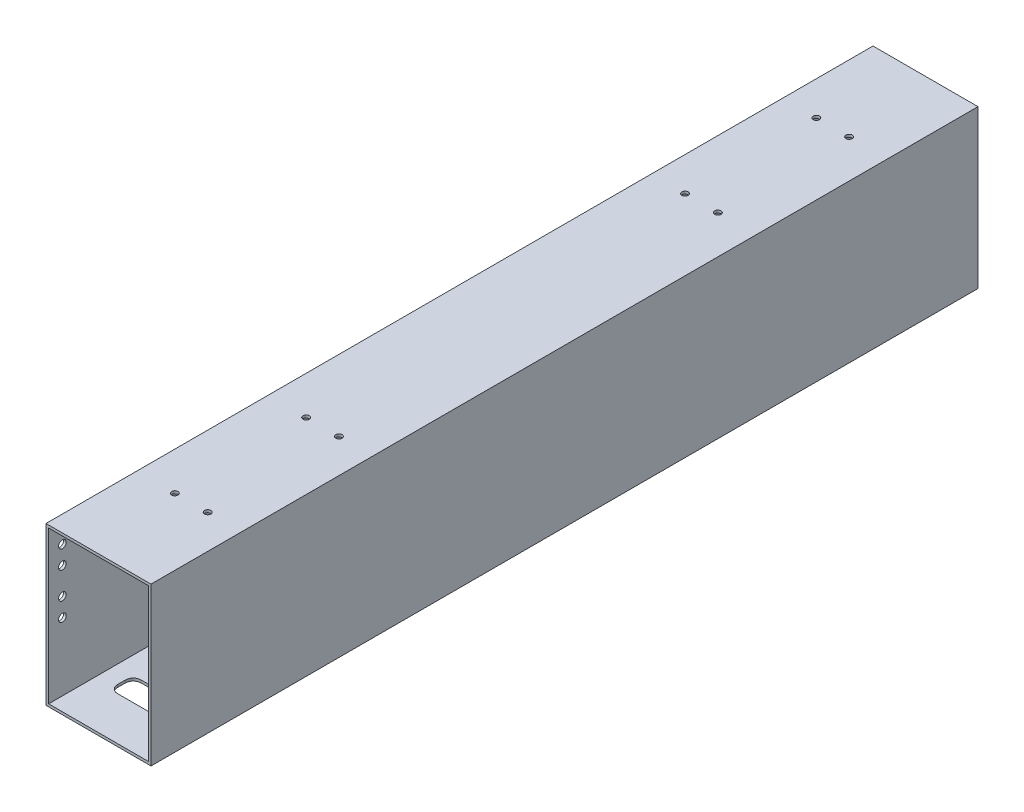
from build123d import *

# Parameters (mm, degrees)
SKETCH_1_W             = 80
SKETCH_1_H             = 120
SKETCH_1_W_2           = 76
SKETCH_1_H_2           = 116
EXTRUDE_1_DEPTH        = 315
CUT_EXTRUDE_2_REACH    = 332.492
SKETCH_4_R             = 25
HOLE_WIZARD_M5_1_D     = 5.8
HOLE_WIZARD_M5_1_DEPTH = 2
HOLE_WIZARD_M4_1_D     = 4.8
HOLE_WIZARD_M4_1_DEPTH = 2
CUT_EXTRUDE_3_REACH    = 341.448
SKETCH_15_W            = 50
SKETCH_15_H            = 18
SKETCH_15_W_2          = 60
SKETCH_15_H_2          = 75
FILLET_1_R             = 6


with BuildPart() as part:
    # 草图1 → 拉伸-薄壁1 (new, symmetric)
    with BuildSketch(Plane.XY):
        Rectangle(SKETCH_1_W, SKETCH_1_H)
        Rectangle(SKETCH_1_W_2, SKETCH_1_H_2, mode=Mode.SUBTRACT)
    extrude(amount=EXTRUDE_1_DEPTH, both=True)

    # 草图4 → 切除-拉伸2 (cut, up to next)
    with BuildSketch(Plane.ZY.offset(40), mode=Mode.PRIVATE) as cut_extrude_2_sk1:
        with Locations((0, -20)):
            Circle(SKETCH_4_R)
    cut_extrude_2_tool1 = extrude(cut_extrude_2_sk1.sketch, amount=-CUT_EXTRUDE_2_REACH, mode=Mode.PRIVATE) & part.part
    add(cut_extrude_2_tool1.solids().sort_by_distance((-40, -20, 0))[0], mode=Mode.SUBTRACT)

    # M5 间隙孔1
    with Locations(Plane.ZY.offset(40)):
        with Locations((304.5, 42), (304.5, 28), (304.5, 7.61), (304.5, -6.39), (-304.5, -6.39), (-304.5, 7.61), (-304.5, 28), (-304.5, 42)):
            Hole(HOLE_WIZARD_M5_1_D / 2, depth=HOLE_WIZARD_M5_1_DEPTH)

    # M4 间隙孔1
    with Locations(Plane(origin=(0, 60, 0), x_dir=(1, 0, 0), z_dir=(0, 1, 0))):
        with Locations((-14.175, 246), (10.825, 246), (-14.175, 146), (10.825, 146), (-10.825, -146), (14.175, -146), (-10.825, -246), (14.175, -246)):
            Hole(HOLE_WIZARD_M4_1_D / 2, depth=HOLE_WIZARD_M4_1_DEPTH)

    # 草图15 → 切除-拉伸3 (cut, up to next)
    with BuildSketch(Plane.XZ.offset(60), mode=Mode.PRIVATE) as cut_extrude_3_sk1:
        with Locations((0.475, -273)):
            Rectangle(SKETCH_15_W, SKETCH_15_H)
    cut_extrude_3_tool1 = extrude(cut_extrude_3_sk1.sketch, amount=-CUT_EXTRUDE_3_REACH, mode=Mode.PRIVATE) & part.part
    # 草图15 → 切除-拉伸3 (cut, up to next)
    with BuildSketch(Plane.XZ.offset(60), mode=Mode.PRIVATE) as cut_extrude_3_sk2:
        with Locations((1.975, -171.5)):
            Rectangle(SKETCH_15_W_2, SKETCH_15_H_2)
    cut_extrude_3_tool2 = extrude(cut_extrude_3_sk2.sketch, amount=-CUT_EXTRUDE_3_REACH, mode=Mode.PRIVATE) & part.part
    # 草图15 → 切除-拉伸3 (cut, up to next)
    with BuildSketch(Plane.XZ.offset(60), mode=Mode.PRIVATE) as cut_extrude_3_sk3:
        with Locations((1.975, 171.5)):
            Rectangle(SKETCH_15_W_2, SKETCH_15_H_2)
    cut_extrude_3_tool3 = extrude(cut_extrude_3_sk3.sketch, amount=-CUT_EXTRUDE_3_REACH, mode=Mode.PRIVATE) & part.part
    # 草图15 → 切除-拉伸3 (cut, up to next)
    with BuildSketch(Plane.XZ.offset(60), mode=Mode.PRIVATE) as cut_extrude_3_sk4:
        with Locations((0.475, 273)):
            Rectangle(SKETCH_15_W, SKETCH_15_H)
    cut_extrude_3_tool4 = extrude(cut_extrude_3_sk4.sketch, amount=-CUT_EXTRUDE_3_REACH, mode=Mode.PRIVATE) & part.part
    add(cut_extrude_3_tool1.solids().sort_by_distance((0.475, -60, -273))[0], mode=Mode.SUBTRACT)
    add(cut_extrude_3_tool2.solids().sort_by_distance((1.975, -60, -171.5))[0], mode=Mode.SUBTRACT)
    add(cut_extrude_3_tool3.solids().sort_by_distance((1.975, -60, 171.5))[0], mode=Mode.SUBTRACT)
    add(cut_extrude_3_tool4.solids().sort_by_distance((0.475, -60, 273))[0], mode=Mode.SUBTRACT)

    # 圆角1
    fillet_1_edges = [part.edges().sort_by_distance(p)[0] for p in [
        (25.475, -59, -282),
        (25.475, -59, -264),
        (-24.525, -59, -264),
        (-24.525, -59, -282),
        (-28.025, -59, 134),
        (31.975, -59, 134),
        (31.975, -59, 209),
        (-28.025, -59, 209),
        (-24.525, -59, 282),
        (-24.525, -59, 264),
        (25.475, -59, 264),
        (25.475, -59, 282),
        (31.975, -59, -209),
        (31.975, -59, -134),
        (-28.025, -59, -134),
        (-28.025, -59, -209),
    ]]
    fillet(fillet_1_edges, radius=FILLET_1_R)


solid = part.part
